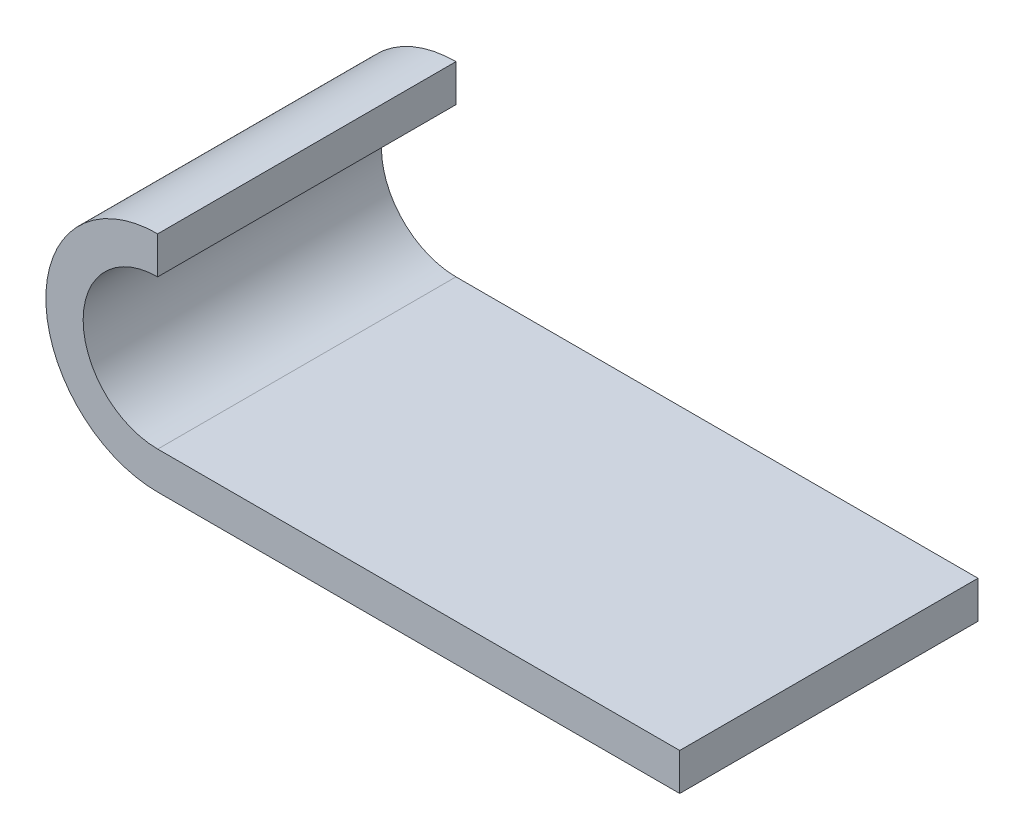
SolidWorks part; units mm, degrees
material "PBT general purpose"
ref_plane "Front Plane" through (0, 0, 0) normal (0, 0, 1) x (1, 0, 0)
ref_plane "Top Plane" through (0, 0, 0) normal (0, 1, 0) x (1, 0, 0)
ref_plane "Right Plane" through (0, 0, 0) normal (1, 0, 0) x (0, 0, -1)
sketch "Sketch1" plane through (0, 0, 0) normal (0, 0, 1) x (1, 0, 0)
  line L0 (-1.5383, -40.5073) -> (-15.5383, -40.5073)
  line L1 (-1.5383, -41.5073) -> (-15.5383, -41.5073)
  line L2 (-15.5383, -35.5073) -> (-15.5383, -36.5073)
  line L3 (-1.5383, -40.5073) -> (-1.5383, -41.5073)
  arc A0 (-15.5383, -36.5073) -> (-15.5383, -40.5073) centre (-15.5383, -38.5073) ccw
  arc A1 (-15.5383, -35.5073) -> (-15.5383, -41.5073) centre (-15.5383, -38.5073) ccw
  dimension "D1" = 1
extrude "Boss-Extrude1" add sketch "Sketch1" along normal blind 8
